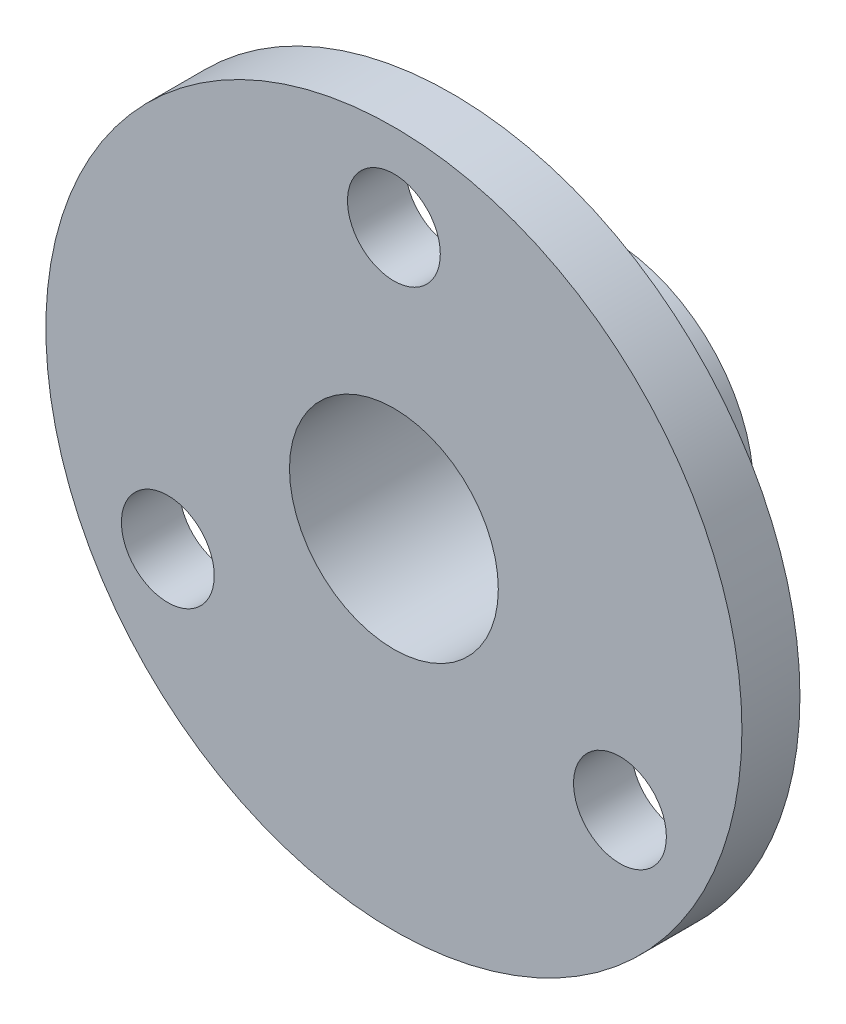
from build123d import *
from build123d.topology import SkipClean

# Parameters (mm, degrees)
SKETCH_1_R      = 30
SKETCH_1_R_2    = 9
SKETCH_1_R_3    = 4
EXTRUDE_1_DEPTH = 5
EXTRUDE_START   = 10
SKETCH_2_R      = 14
SKETCH_2_R_2    = 9
EXTRUDE_2_DEPTH = 10
SKETCH_3_R      = 12.5
SKETCH_3_R_2    = 8.1
EXTRUDE_3_DEPTH = 3.5


with BuildPart() as part:
    # 草图1 → 凸台-拉伸1 (new body)
    with BuildSketch(Plane.XY):
        Circle(SKETCH_1_R)
        Circle(SKETCH_1_R_2, mode=Mode.SUBTRACT)
        with Locations((0, 22.5)):
            Circle(SKETCH_1_R_3, mode=Mode.SUBTRACT)
        with Locations((19.485571585, -11.25)):
            Circle(SKETCH_1_R_3, mode=Mode.SUBTRACT)
        with Locations((-19.485571585, -11.25)):
            Circle(SKETCH_1_R_3, mode=Mode.SUBTRACT)
    extrude(amount=EXTRUDE_1_DEPTH)

    # 草图2 → 凸台-拉伸2 (add)
    with SkipClean():  # the faces are left unmerged after this step: merging them gives an invalid solid
        with BuildSketch(Plane(origin=(0, 0, 0), x_dir=(-1, 0, 0), z_dir=(0, 0, -1)).offset(EXTRUDE_START)):
            with Locations(Location((0, 0, 0), (0, 0, 180))):
                Circle(SKETCH_2_R)
            Circle(SKETCH_2_R_2, mode=Mode.SUBTRACT)
        extrude(amount=-EXTRUDE_2_DEPTH)

    # 草图3 → 凸台-拉伸3 (add)
    with SkipClean():  # the faces are left unmerged after this step: merging them gives an invalid solid
        with BuildSketch(Plane(origin=(0, 0, -10), x_dir=(-1, 0, 0), z_dir=(0, 0, -1))):
            Circle(SKETCH_3_R)
            Circle(SKETCH_3_R_2, mode=Mode.SUBTRACT)
        extrude(amount=EXTRUDE_3_DEPTH)


solid = part.part
